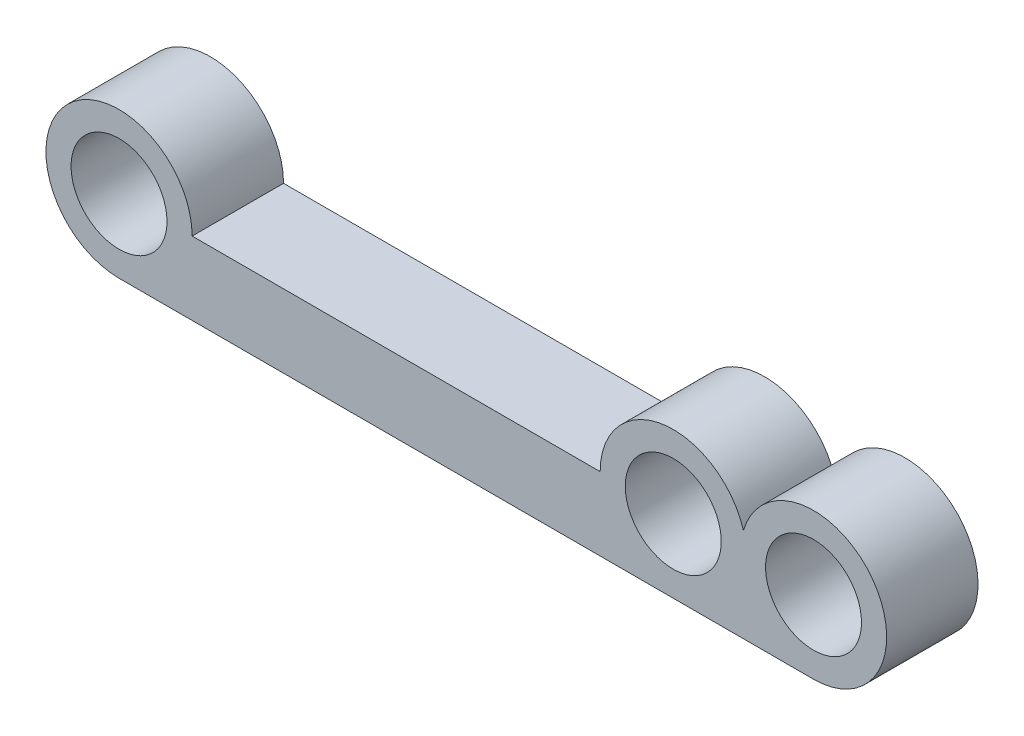
SolidWorks part; units mm, degrees
ref_plane "Front Plane" through (0, 0, 0) normal (0, 0, 1) x (1, 0, 0)
ref_plane "Top Plane" through (0, 0, 0) normal (0, 1, 0) x (1, 0, 0)
ref_plane "Right Plane" through (0, 0, 0) normal (1, 0, 0) x (0, 0, -1)
other "Configuration Table"
sketch "Sketch1" plane through (0, 0, 0) normal (0, 0, 1) x (1, 0, 0)
  line L1 (1, 0) -> (44, 0)
  line L2 (0, -1) -> (0, -4)
  line L3 (1, -5) -> (44, -5)
  line L4 (45, -1) -> (45, -4)
  arc A0 (45, -1) -> (44, 0) centre (44, -1) ccw
  arc A1 (44, -5) -> (45, -4) centre (44, -4) ccw
  arc A2 (0, -1) -> (1, 0) centre (1, -1) cw
  arc A3 (0, -4) -> (1, -5) centre (1, -4) ccw
  point P7 (45, 0)
  point P12 (0, 0)
  point P15 (0, -5)
extrude "Boss-Extrude1" add sketch "Sketch1" along normal blind 5
sketch "Sketch2" plane through (0, 0, 0) normal (0, 0, -1) x (-1, 0, 0)
  line L0 (-45, -2.5) -> (0, -2.5) construction
  line L1 (-45, -4) -> (-45, -1) construction
  line L2 (0, -1) -> (0, -4) construction
  line L3 (-45, -2.5) -> (-42.676, -2.5) construction
  line L4 (-45, -2.5) -> (-42.676, -2.5) construction
  circle A0 centre (-42.676, -2.5) radius 2.5
extrude "Boss-Extrude2" add sketch "Sketch2" along normal blind 7
sketch "Sketch3" plane through (0, 0, 5) normal (0, 0, 1) x (1, 0, 0)
  line L0 (45, -2.5) -> (0, -2.5) construction
  line L1 (45, -4) -> (45, -1) construction
  line L2 (0, -1) -> (0, -4) construction
sketch "Sketch4" plane through (0, 0, 5) normal (0, 0, 1) x (1, 0, 0)
  line L0 (45, -2.5) -> (35, -2.5) construction
  line L1 (45, -4) -> (45, -1) construction
  circle A0 centre (35, -2.5) radius 2.5
extrude "Boss-Extrude4" add sketch "Sketch4" along normal blind 9
sketch "Sketch9" plane through (0, 0, 0) normal (0, 0, -1) x (-1, 0, 0)
  line L0 (-42.676, -2.5) -> (-4.676, -2.5) construction
  line L1 (-45, -2.5) -> (0, -2.5) construction
sketch "Sketch10" plane through (0, 0, 5) normal (0, 0, 1) x (1, 0, 0)
  circle A0 centre (4.676, -2.5) radius 2.5
extrude "Boss-Extrude6" add sketch "Sketch10" along normal blind 5
sketch "Sketch11" plane through (0, 0, 0) normal (0, 0, -1) x (-1, 0, 0)
  line L0 (-42.676, -2.5) -> (-4.676, -2.5) construction
sketch "Sketch12" plane through (0, 0, 14) normal (0, 0, 1) x (1, 0, 0)
  line L0 (35, -2.5) -> (35, 0) construction
  circle A0 centre (35, -2.5) radius 2.5 construction
  circle A1 centre (35, -2.5) radius 2.5 construction
ref_plane "Plane1"
sketch "Sketch13" plane through (35, 0, 1.9958) normal (1, 0, 0) x (0, 1, 0)
  line L2 (0, 8.75) -> (-0.75, 8.75)
  line L3 (-0.75, 8.75) -> (-0.75, 8)
  line L4 (-0.75, 8) -> (0, 8)
  line L5 (0, 8) -> (0, 8.75)
  line L6 (-2.5, 14) -> (-2.5, 6.7417) construction
  line L8 (-5, 8) -> (-5, 8.75)
  line L9 (-4.25, 8) -> (-5, 8)
  line L10 (-4.25, 8.75) -> (-4.25, 8)
  line L11 (-5, 8.75) -> (-4.25, 8.75)
revolve "Cut-Revolve1" cut sketch "Sketch13" angle 45 about L6 other way angle 45
sketch "Sketch14" plane through (0, 0, -7) normal (0, 0, -1) x (-1, 0, 0)
  line L0 (-42.676, -2.5) -> (-42.676, 0) construction
  circle A0 centre (-42.676, -2.5) radius 2.5 construction
  circle A1 centre (-42.676, -2.5) radius 2.5 construction
ref_plane "Plane2"
sketch "Sketch15" plane through (42.676, 0, -1.9999) normal (-1, 0, 0) x (0, 1, 0)
  line L2 (0, 3.75) -> (-0.75, 3.75)
  line L3 (-0.75, 3.75) -> (-0.75, 3)
  line L4 (-0.75, 3) -> (0, 3)
  line L5 (0, 3) -> (0, 3.75)
  line L6 (-2.5, 7) -> (-2.5, 3.2255) construction
  line L10 (-5, 3) -> (-5, 3.75)
  line L11 (-4.25, 3) -> (-5, 3)
  line L12 (-4.25, 3.75) -> (-4.25, 3)
  line L13 (-5, 3.75) -> (-4.25, 3.75)
revolve "Cut-Revolve2" cut sketch "Sketch15" angle 45 about L6 other way angle 45
sketch "Sketch17" plane through (0, 0, 5) normal (0, 0, 1) x (1, 0, 0)
  circle A0 centre (42.676, -2.5) radius 4
extrude "Boss-Extrude7" add sketch "Sketch17" against normal blind 5
sketch "Sketch18" plane through (0, 0, -7) normal (0, 0, -1) x (-1, 0, 0)
  circle A0 centre (-42.676, -2.5) radius 2.9309
extrude "Cut-Extrude1" cut sketch "Sketch18" against normal blind 7
sketch "Sketch19" plane through (0, 0, 5) normal (0, 0, 1) x (1, 0, 0)
  circle A0 centre (42.676, -2.5) radius 2.625
extrude "Cut-Extrude2" cut sketch "Sketch19" against normal blind 7
sketch "Sketch20" plane through (0, 0, 0) normal (0, 0, -1) x (-1, 0, 0)
  circle A0 centre (-35, -2.5) radius 4
extrude "Boss-Extrude8" add sketch "Sketch20" against normal blind 5
sketch "Sketch21" plane through (0, 0, 0) normal (0, 0, -1) x (-1, 0, 0)
  circle A0 centre (-35, -2.5) radius 2.625
extrude "Cut-Extrude3" cut sketch "Sketch21" against normal through all
sketch "Sketch23" plane through (0, 0, 5) normal (0, 0, 1) x (1, 0, 0)
  circle A0 centre (4.676, -2.5) radius 4
extrude "Boss-Extrude9" add sketch "Sketch23" against normal blind 5
sketch "Sketch24" plane through (0, 0, 10) normal (0, 0, 1) x (1, 0, 0)
  circle A0 centre (4.676, -2.5) radius 2.625
extrude "Cut-Extrude4" cut sketch "Sketch24" against normal blind 15
sketch "Sketch25" plane through (0, 0, 5) normal (0, 0, 1) x (1, 0, 0)
  line L0 (1, -5) -> (1.5536, -5) construction
  line L1 (1.5536, -5) -> (-1.8547, -7.7288)
  line L2 (-1.8547, -7.7288) -> (-3.4365, -2.8749)
  line L3 (-3.4365, -2.8749) -> (-1.5365, 1.5938)
  line L4 (-1.5365, 1.5938) -> (0.676, 3.0378)
  line L5 (0.676, 3.0378) -> (1.5536, 0)
  arc A0 (1.5536, 0) -> (1.5536, -5) centre (4.676, -2.5) ccw
extrude "Cut-Extrude5" cut sketch "Sketch25" against normal blind 10
sketch "Sketch26" plane through (0, 0, 5) normal (0, 0, 1) x (1, 0, 0)
  line L0 (45, -2.5) -> (0, -2.5) construction
  line L1 (31.8775, 0) -> (7.7985, 0) construction
  line L2 (8.676, -2.5) -> (31, -2.5)
  line L3 (31, 2.8838) -> (31, 2.9101)
  line L4 (31, 2.9101) -> (31.8775, 0)
  line L5 (31, 2.8838) -> (7.7985, 0)
  line L6 (38.1225, 0) -> (39.4037, 2.5424)
  line L7 (39.4037, 2.5424) -> (39.8662, 0.3469)
  arc A0 (7.7985, 0) -> (8.676, -2.5) centre (4.676, -2.5) cw
  arc A1 (31.8775, 0) -> (31, -2.5) centre (35, -2.5) ccw
  arc A2 (38.1225, 0) -> (39, -2.5) centre (35, -2.5) cw
  arc A3 (39.8662, 0.3469) -> (38.838, -1.3732) centre (42.676, -2.5) ccw
  arc A4 (39.5536, -5) -> (39.5536, 0) centre (42.676, -2.5) ccw construction
  line M1 (31.8775, 0) -> (7.7985, 0)
  arc M6 (39.5536, -5) -> (39.5536, 0) centre (42.676, -2.5) ccw
  line M7 (39.5536, 0) -> (38.1225, 0)
extrude "Cut-Extrude6" cut sketch "Sketch26" against normal through all contours L3 L5 L4 M1 | L7 L6 M7 M6 | A1 A0 L2 M1 | A3 A2 M7
sketch "Sketch27" plane through (0, 0, 5) normal (0, 0, 1) x (1, 0, 0)
  line L0 (4.676, -6.5) -> (35, -6.5)
  line L1 (35, -6.5) -> (42.676, -6.5)
  line L2 (42.676, -6.5) -> (39.4291, -3.9663)
  line L3 (39.4291, -3.9663) -> (35, -5.9665)
  line L4 (35, -5.9665) -> (31.2871, -3.9663)
  line L5 (31.2871, -3.9663) -> (8.2888, -3.9663)
  line L6 (8.2888, -3.9663) -> (4.676, -6.5)
  arc A0 (8.676, -2.5) -> (7.7985, -5) centre (4.676, -2.5) ccw construction
  arc A1 (31.8775, -5) -> (38.1225, -5) centre (35, -2.5) ccw construction
  arc A2 (39.5536, -5) -> (38.838, -1.3732) centre (42.676, -2.5) ccw construction
extrude "Boss-Extrude10" add sketch "Sketch27" against normal through all
